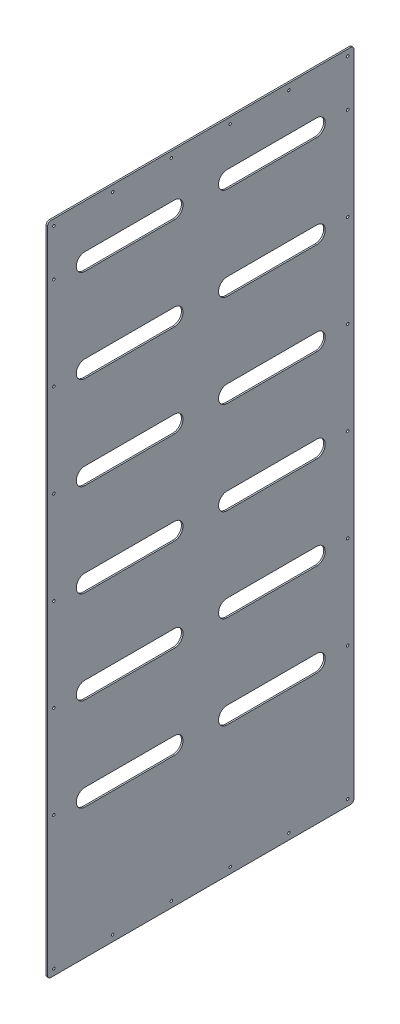
from build123d import *

# Parameters (mm, degrees)
SKETCH1_W                     = 990
SKETCH1_H                     = 2120
BOSS_EXTRUDE1_DEPTH           = 5
FILLET1_R                     = 10
M7_CLEARANCE_HOLE3_D          = 8
M7_CLEARANCE_HOLE2_AT_2_COUNT = 2
M7_CLEARANCE_HOLE2_AT_2_PITCH = 950
LPATTERN7_COUNT               = 6
LPATTERN7_PITCH               = 300
CUT_EXTRUDE5_DEPTH            = 10
LPATTERN8_COUNT               = 6
LPATTERN8_PITCH               = 300
MIRROR6_COPY_1_DEPTH          = 10
MIRROR6_COPY_2_DEPTH          = 10
MIRROR6_COPY_3_DEPTH          = 10
MIRROR6_COPY_4_DEPTH          = 10
MIRROR6_COPY_5_DEPTH          = 10


with BuildPart() as part:
    # Sketch1 → Boss-Extrude1 (new body)
    with BuildSketch(Plane(origin=(0, 0, 0), x_dir=(0, 0, -1), z_dir=(1, 0, 0))):
        Rectangle(SKETCH1_W, SKETCH1_H)
    extrude(amount=BOSS_EXTRUDE1_DEPTH)

    # Fillet1
    fillet1_edges = [part.edges().sort_by_distance(p)[0] for p in [
        (2.5, -1060, -495),
        (2.5, -1060, 495),
        (2.5, 1060, 495),
        (2.5, 1060, -495),
    ]]
    fillet(fillet1_edges, radius=FILLET1_R)

    # M7 Clearance Hole3 (through all)
    with Locations(Plane(origin=(5, 0, 0), x_dir=(0, 0, -1), z_dir=(1, 0, 0))):
        with Locations((-475, 1040), (-285, 1040), (-95, 1040), (95, 1040), (285, 1040), (475, 1040)):
            m7_clearance_hole3 = Hole(M7_CLEARANCE_HOLE3_D / 2)

    # Mirror5: M7 Clearance Hole3 across plane
    add(m7_clearance_hole3.mirror(Plane(origin=(0, 0, 0), x_dir=(0, 0, 1), z_dir=(0, -1, 0))), mode=Mode.SUBTRACT)

    # Sketch15 → M7 Clearance Hole2 (revolve, cut)
    with BuildSketch(Plane(origin=(5, 890, 475), x_dir=(0, 0, -1), z_dir=(0, 1, 0))):
        Polygon((0, 0), (0, 7.403442476), (4, 5), (4, 0), align=None)
    m7_clearance_hole2 = revolve(axis=Axis((11.35, 890, 475), (-1, 0, 0)), mode=Mode.SUBTRACT)

    # M7 Clearance Hole2 at 2: M7 Clearance Hole2 ×2
    with Locations(*[(0, 0, -i * M7_CLEARANCE_HOLE2_AT_2_PITCH) for i in range(1, M7_CLEARANCE_HOLE2_AT_2_COUNT)]):
        add(m7_clearance_hole2, mode=Mode.SUBTRACT)

    # LPattern7: M7 Clearance Hole2 ×6
    with Locations(*[(0, -i * LPATTERN7_PITCH, 0) for i in range(1, LPATTERN7_COUNT)]):
        add(m7_clearance_hole2, mode=Mode.SUBTRACT)

    # LPattern7 copy 1 sketch → LPattern7 copy 1 (revolve, cut)
    with BuildSketch(Plane(origin=(5, 590, -475), x_dir=(0, 0, -1), z_dir=(0, 1, 0))):
        Polygon((0, 0), (0, 7.403442476), (4, 5), (4, 0), align=None)
    revolve(axis=Axis((11.35, 590, -475), (-1, 0, 0)), mode=Mode.SUBTRACT)

    # LPattern7 copy 2 sketch → LPattern7 copy 2 (revolve, cut)
    with BuildSketch(Plane(origin=(5, 290, -475), x_dir=(0, 0, -1), z_dir=(0, 1, 0))):
        Polygon((0, 0), (0, 7.403442476), (4, 5), (4, 0), align=None)
    revolve(axis=Axis((11.35, 290, -475), (-1, 0, 0)), mode=Mode.SUBTRACT)

    # LPattern7 copy 3 sketch → LPattern7 copy 3 (revolve, cut)
    with BuildSketch(Plane(origin=(5, -10, -475), x_dir=(0, 0, -1), z_dir=(0, 1, 0))):
        Polygon((0, 0), (0, 7.403442476), (4, 5), (4, 0), align=None)
    revolve(axis=Axis((11.35, -10, -475), (-1, 0, 0)), mode=Mode.SUBTRACT)

    # LPattern7 copy 4 sketch → LPattern7 copy 4 (revolve, cut)
    with BuildSketch(Plane(origin=(5, -310, -475), x_dir=(0, 0, -1), z_dir=(0, 1, 0))):
        Polygon((0, 0), (0, 7.403442476), (4, 5), (4, 0), align=None)
    revolve(axis=Axis((11.35, -310, -475), (-1, 0, 0)), mode=Mode.SUBTRACT)

    # LPattern7 copy 5 sketch → LPattern7 copy 5 (revolve, cut)
    with BuildSketch(Plane(origin=(5, -610, -475), x_dir=(0, 0, -1), z_dir=(0, 1, 0))):
        Polygon((0, 0), (0, 7.403442476), (4, 5), (4, 0), align=None)
    revolve(axis=Axis((11.35, -610, -475), (-1, 0, 0)), mode=Mode.SUBTRACT)

    # Sketch18 → Cut-Extrude5 (cut)
    with BuildSketch(Plane(origin=(5, 0, 0), x_dir=(0, 0, -1), z_dir=(1, 0, 0))):
        with BuildLine():
            Line((-375, 917.5), (-85, 917.5))
            ThreePointArc((-85, 917.5), (-57.5, 890), (-85, 862.5))
            Line((-85, 862.5), (-375, 862.5))
            ThreePointArc((-375, 862.5), (-402.5, 890), (-375, 917.5))
        make_face()
    cut_extrude5 = extrude(amount=-CUT_EXTRUDE5_DEPTH, mode=Mode.SUBTRACT)

    # LPattern8: Cut-Extrude5 ×6
    with Locations(*[(0, -i * LPATTERN8_PITCH, 0) for i in range(1, LPATTERN8_COUNT)]):
        add(cut_extrude5, mode=Mode.SUBTRACT)

    # Mirror6: Cut-Extrude5 across plane
    add(cut_extrude5.mirror(Plane.XY), mode=Mode.SUBTRACT)

    # Mirror6 copy 1 sketch → Mirror6 copy 1 (cut)
    with BuildSketch(Plane(origin=(5, -300, 0), x_dir=(0, 0, 1), z_dir=(1, 0, 0))):
        with BuildLine():
            Line((-375, -917.5), (-85, -917.5))
            ThreePointArc((-85, -917.5), (-57.5, -890), (-85, -862.5))
            Line((-85, -862.5), (-375, -862.5))
            ThreePointArc((-375, -862.5), (-402.5, -890), (-375, -917.5))
        make_face()
    extrude(amount=-MIRROR6_COPY_1_DEPTH, mode=Mode.SUBTRACT)

    # Mirror6 copy 2 sketch → Mirror6 copy 2 (cut)
    with BuildSketch(Plane(origin=(5, -600, 0), x_dir=(0, 0, 1), z_dir=(1, 0, 0))):
        with BuildLine():
            Line((-375, -917.5), (-85, -917.5))
            ThreePointArc((-85, -917.5), (-57.5, -890), (-85, -862.5))
            Line((-85, -862.5), (-375, -862.5))
            ThreePointArc((-375, -862.5), (-402.5, -890), (-375, -917.5))
        make_face()
    extrude(amount=-MIRROR6_COPY_2_DEPTH, mode=Mode.SUBTRACT)

    # Mirror6 copy 3 sketch → Mirror6 copy 3 (cut)
    with BuildSketch(Plane(origin=(5, -900, 0), x_dir=(0, 0, 1), z_dir=(1, 0, 0))):
        with BuildLine():
            Line((-375, -917.5), (-85, -917.5))
            ThreePointArc((-85, -917.5), (-57.5, -890), (-85, -862.5))
            Line((-85, -862.5), (-375, -862.5))
            ThreePointArc((-375, -862.5), (-402.5, -890), (-375, -917.5))
        make_face()
    extrude(amount=-MIRROR6_COPY_3_DEPTH, mode=Mode.SUBTRACT)

    # Mirror6 copy 4 sketch → Mirror6 copy 4 (cut)
    with BuildSketch(Plane(origin=(5, -1200, 0), x_dir=(0, 0, 1), z_dir=(1, 0, 0))):
        with BuildLine():
            Line((-375, -917.5), (-85, -917.5))
            ThreePointArc((-85, -917.5), (-57.5, -890), (-85, -862.5))
            Line((-85, -862.5), (-375, -862.5))
            ThreePointArc((-375, -862.5), (-402.5, -890), (-375, -917.5))
        make_face()
    extrude(amount=-MIRROR6_COPY_4_DEPTH, mode=Mode.SUBTRACT)

    # Mirror6 copy 5 sketch → Mirror6 copy 5 (cut)
    with BuildSketch(Plane(origin=(5, -1500, 0), x_dir=(0, 0, 1), z_dir=(1, 0, 0))):
        with BuildLine():
            Line((-375, -917.5), (-85, -917.5))
            ThreePointArc((-85, -917.5), (-57.5, -890), (-85, -862.5))
            Line((-85, -862.5), (-375, -862.5))
            ThreePointArc((-375, -862.5), (-402.5, -890), (-375, -917.5))
        make_face()
    extrude(amount=-MIRROR6_COPY_5_DEPTH, mode=Mode.SUBTRACT)


solid = part.part
